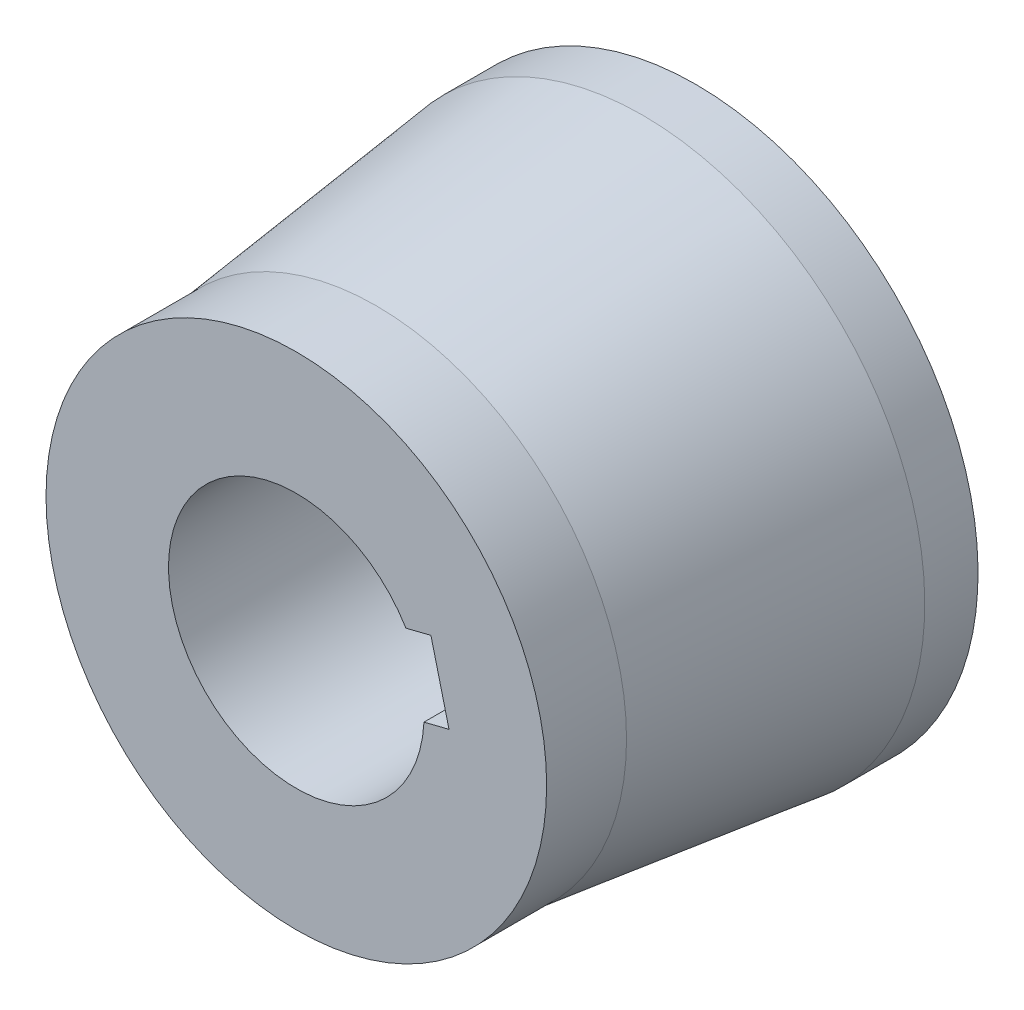
SolidWorks part; units mm, degrees
ref_plane "Front Plane" through (0, 0, 0) normal (0, 0, 1) x (1, 0, 0)
ref_plane "Top Plane" through (0, 0, 0) normal (0, 1, 0) x (1, 0, 0)
ref_plane "Right Plane" through (0, 0, 0) normal (1, 0, 0) x (0, 0, -1)
ref_plane "Plane1" through (0, 234.744, 0) normal (0, -1, 0) x (1, 0, 0)
sketch "Sketch1" plane through (0, 234.744, 0) normal (0, -1, 0) x (1, 0, 0)
  line L0 (568.2306, -1074.9984) -> (521.2306, -1074.9984)
  line L1 (521.2306, -1074.9984) -> (521.2306, -1149.9984)
  line L2 (521.2306, -1149.9984) -> (574.2306, -1149.9984)
  line L3 (574.2306, -1149.9984) -> (574.2306, -1139.9984)
  line L4 (574.2306, -1139.9984) -> (568.2306, -1089.9984)
  line L5 (568.2306, -1089.9984) -> (568.2306, -1074.9984)
  line L6 (521.2306, -1074.9984) -> (521.2306, -1149.9984) construction
  dimension "D1" = 47
  dimension "D2" = 53
  dimension "D3" = 10
  dimension "D4" = 60
  dimension "D5" = 75
revolve "Revolve1" add sketch "Sketch1" angle 360 about L6
sketch "Sketch2" plane through (0, 0, -1074.9984) normal (0, 0, 1) x (1, 0, 0)
  line L0 (549.8983, 234.6929) -> (546.5041, 248.2752)
  line L1 (546.5041, 248.2752) -> (541.8051, 247.1009)
  line L2 (545.1993, 233.5186) -> (549.8983, 234.6929)
  arc A0 (541.8051, 247.1009) -> (545.1993, 233.5186) centre (521.2306, 234.744) cw
  circle A1 centre (521.2306, 234.744) radius 47 construction
  dimension "D1" = 24
  dimension "D2" = 20.5744
  dimension "D3" = 23.9687
  dimension "D4" = 25.2734
  dimension "D5" = 28.6677
  dimension "D6" = 12.3569
  dimension "D7" = 13.5312
  dimension "D8" = 0.0511
  dimension "D9" = 1.2254
extrude "Cut-Extrude1" cut sketch "Sketch2" against normal through all
sketch "Sketch3" plane through (0, 234.744, 0) normal (0, -1, 0) x (1, 0, 0)
  line L0 (545.2306, -1074.9984) -> (521.2306, -1074.9984)
  line L1 (521.2306, -1074.9984) -> (521.2306, -1149.9984)
  line L2 (521.2306, -1149.9984) -> (545.2306, -1149.9984)
  line L3 (545.2306, -1149.9984) -> (545.2306, -1074.9984)
  line L4 (521.2306, -1074.9984) -> (521.2306, -1149.9984) construction
  dimension "D1" = 24
  dimension "D2" = 75
revolve "Cut-Revolve1" cut sketch "Sketch3" angle 360 about L4
